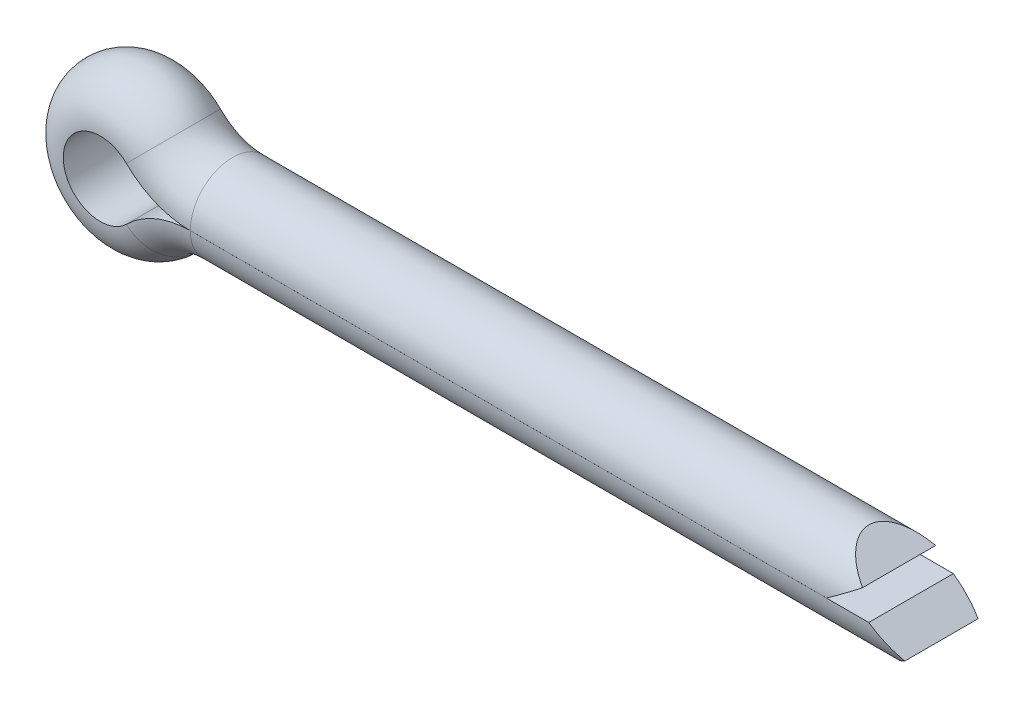
from build123d import *

# Parameters (mm, degrees)
CONECUT_DEPTH      = 68.537026869
CONECUT_DEPTH_BACK = 68.537026869


with BuildPart() as part:
    # Body: sweep along a path in 草图2
    with BuildLine(Plane.XY) as body_path:
        Line((63, 4), (0, 4))
        ThreePointArc((0, 4), (-1.740570538, 4.344328693), (-3.218934911, 5.325443787))
        ThreePointArc((-3.218934911, 5.325443787), (-16, 0), (-3.218934911, -5.325443787))
        ThreePointArc((-3.218934911, -5.325443787), (-1.740570538, -4.344328693), (0, -4))
        Line((0, -4), (67, -4))
    # 草图1 → Body (sweep)
    with BuildSketch(Plane(origin=(63, 0, 0), x_dir=(0, 0, -1), z_dir=(1, 0, 0))):
        with BuildLine():
            Line((-3.9999995, 0.002), (3.9999995, 0.002))
            ThreePointArc((3.9999995, 0.002), (0, 4), (-3.9999995, 0.002))
        make_face()
    sweep(path=body_path.line)

    # 草图3 → ConeCut (cut, two sides: drawn at the far end of the back side and taken through both)
    with BuildSketch(Plane.XY.offset(-CONECUT_DEPTH_BACK)):
        Polygon((63, 2.001), (60.139364077, 4.01), (67.01, 4.01), (67.01, -4.01), (64.139364077, -4.01), (67, -2.001), (64.133762416, 0), (60.133762416, 0), align=None)
    extrude(amount=CONECUT_DEPTH + CONECUT_DEPTH_BACK, mode=Mode.SUBTRACT)


solid = part.part
